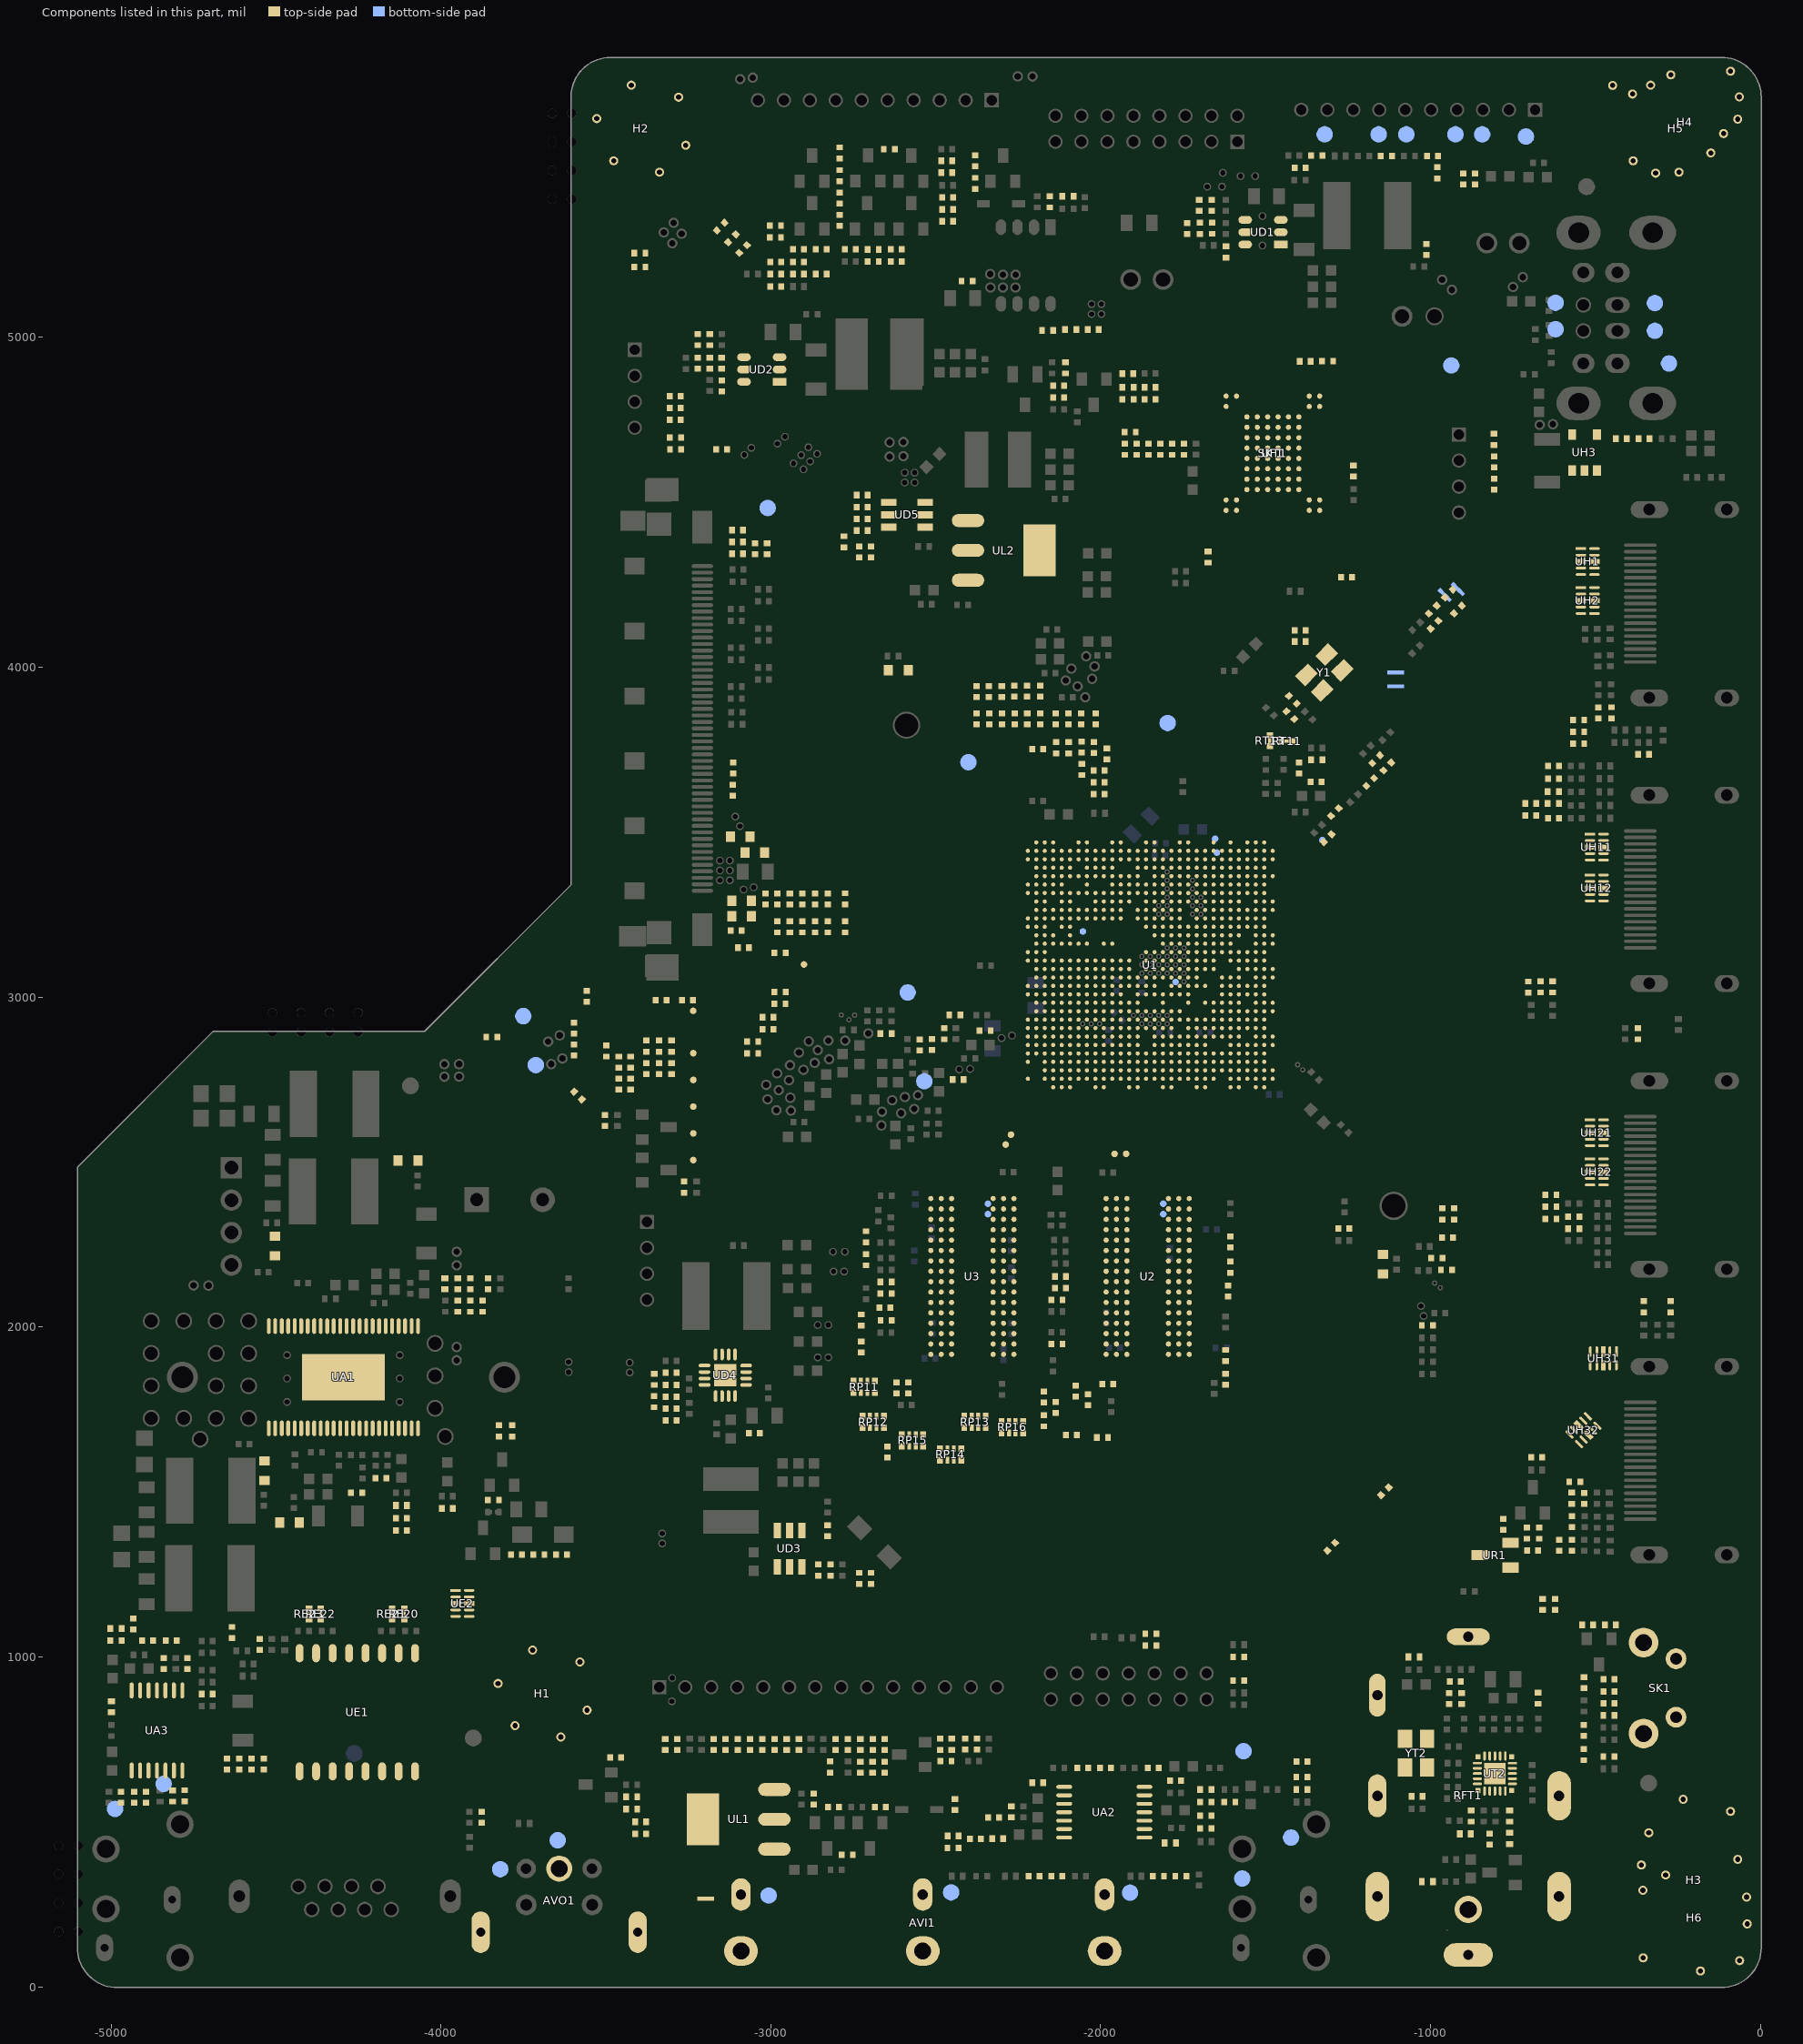
[diagram p0: the components of this part, seen from the top]
# Altium PCB MISC86290.PcbDoc (part 4 of 31)
Units mil, origin at the board's own origin, x right, y up, seen from the top; angles counter-clockwise.
Board outline 5104.71 x 5851.49 mil, 2 copper layers (TopLayer, BottomLayer), stack 61.855 mil thick; 1026 components, 667 nets, 4280 pads, 2294 vias.

## Components (designator, comment, footprint, x,y, rotation, side; value= is the part's Value field where it differs from the comment) (continued)
RE3 "75ohm-0402-±1%-1/16W" R0402 -4611.33,675.23 r270 top
RE4 "75ohm-0402-±1%-1/16W" R0402 -4648.5,675.23 r270 top
RE6 "0ohm-0402-±5%-1/16W" R0402 -4549.6,1037.94 r270 top
RE20 "NC/0ohm-0402-PCB" R0402SC -4111.5,1130.02 r270 top
RE21 "NC/0ohm-0402-PCB" R0402SC -4148.5,1130.02 r270 top
RE22 "NC/0ohm-0402-PCB" R0402SC -4364.5,1130.02 r270 top
RE23 "NC/0ohm-0402-PCB" R0402SC -4400,1130.02 r270 top
RF1 "Thick-film resistor,RES,1/16W,1Kohm,±5%,0402,SMD" R0402 -1910.52,4713.11 r180 top
RF2 "Thick-film resistor,RES,1/16W,3.9Kohm,±1%,0402,SMD" R0402 -1234,4594.77 r270 top
RF3 "0ohm-0402-±5%-1/16W" R0402 -1783.25,4660.84 r90 top
RF4 "0ohm-0402-±5%-1/16W" R0402 -1819.25,4660.84 r90 top
RF5 "0ohm-0402-±5%-1/16W" R0402 -1891.25,4660.84 r90 top
RF6 "0ohm-0402-±5%-1/16W" R0402 -1747.25,4660.84 r90 top
RF7 "0ohm-0402-±5%-1/16W" R0402 -1855.25,4660.84 r90 top
RF8 "0ohm-0402-±5%-1/16W" R0402 -1927.25,4660.84 r90 top
RF56 "Thick-film resistor,RES,1/16W,300Kohm,±1%,0402,SMD" R0402 -1917.25,4848.95 r180 top
RFT1 "RF shield can,RF SHLED,Single,H,F,T14.5,CH6.3,whole,25.0×14.5×10.0mm,DIP,T-14.5×25×10-F14.5-LHD (integrated),LHD" T-14.5×25×10-F14.5-2 -885.83,98.43 r0 top locked
RG1 "NC/1Kohm-0402-±5%-1/16W" R0402 -2464.25,5352 r0 top
RG2 "NC/4K7ohm-0402-±5%-1/16W" R0402 -2847,5267 r180 top
RG3 "NC/33ohm-0402-±5%-1/16W" R0402 -2464.25,5387.84 r180 top
RG4 "4K7ohm-0402-±5%-1/16W" R0402 -2464.25,5424.84 r0 top
RG5 "100ohm-0402-±5%-1/16W" R0402 -2847,5192 r180 top
RG6 "NC/10Kohm-0402-±5%-1/16W" R0402 -3149.23,4661 r0 top
RG7 "NC/1Kohm-0402-±5%-1/16W" R0402 -2791,5354.5 r270 top
RG8 "NC/10Kohm-0402-±5%-1/16W" R0402 -2689.5,5266.5 r180 top
RG11 "NC/10Kohm-0402-±5%-1/16W" R0402 -2986,5303.5 r180 top
RG12 "NC/1Kohm-0402-±5%-1/16W" R0402 -2620,5230.5 r0 top
RG13 "NC/33ohm-0402-±5%-1/16W" R0402 -2467,5499.5 r0 top
RG14 "4K7ohm-0402-±5%-1/16W" R0402 -2467,5535.5 r180 top
RG15 "100ohm-0402-±5%-1/16W" R0402 -2986,5339.5 r180 top
RG16 "NC/10Kohm-0402-±5%-1/16W" R0402 -3557.76,3002.2 r270 top
RG17 "NC/1Kohm-0402-±5%-1/16W" R0402 -2791,5559.5 r270 top
RG18 "NC/10Kohm-0402-±5%-1/16W" R0402 -2641,5571 r180 top
RG30 "NC/4K7ohm-0402-±5%-1/16W" R0402 -2985,5229 r180 top
RG31 "4K7ohm-0402-±5%-1/16W" R0402 -2916,5192 r180 top
RG32 "NC/100ohm-0402-±5%-1/16W" R0402 -2985,5154 r0 top
RG33 "100ohm-0402-±5%-1/16W" R0402 -2985,5192 r0 top
RG34 "NC/10Kohm-0402-±5%-1/16W" R0402 -2916,5229 r180 top
RG35 "0ohm-0402-±5%-1/16W" R0402 -2916,5267 r180 top
RG36 "NC/10Kohm-0402-±5%-1/16W" R0402 -2791,5422.5 r90 top
RG37 "NC/1Kohm-0402-±5%-1/16W" R0402 -2620,5267 r0 top
RG38 "NC/1Kohm-0402-±5%-1/16W" R0402 -2791,5490.5 r90 top
RG39 "NC/33ohm-0402-±5%-1/16W" R0402 -2689.5,5230 r180 top
RG40 "NC/2K2ohm-0402-±5%-1/16W" R0402 -2759,5267 r0 top
RG41 "100ohm-0402-±5%-1/16W" R0402 -3152,5336 r225 top
RG42 "100ohm-0402-±5%-1/16W" R0402 -3084,5268 r225 top
RG43 "100ohm-0402-±5%-1/16W" R0402 -2972,3134.5 r0 top
RG44 "100ohm-0402-±5%-1/16W" R0402 -3289.27,4696.5 r0 top
RH1 "Thick-film resistor,RES,1/16W,33ohm,±5%,0402,SMD" R0402 -354,3736 r180 top
RH2 "47Kohm-0402-±5%-1/16W" R0402 -451,3862 r270 top
RH3 "47Kohm-0402-±5%-1/16W" R0402 -491,3861.73 r270 top
RH4 "Thick-film resistor,RES,1/16W,33ohm,±5%,0402,SMD" R0402 -551,3768 r0 top
RH5 "100ohm-0402-±5%-1/16W" R0402 -551,3840 r180 top
RH6 "100ohm-0402-±5%-1/16W" R0402 -551,3804 r180 top
RH11 "Thick-film resistor,RES,1/16W,33ohm,±5%,0402,SMD" R0402 -627,3701 r0 top
RH12 "Thick-film resistor,RES,1/16W,33ohm,±5%,0402,SMD" R0402 -627,3662 r0 top
RH13 "47Kohm-0402-±5%-1/16W" R0402 -628,3623 r180 top
RH14 "47Kohm-0402-±5%-1/16W" R0402 -628,3587 r180 top
RH15 "100ohm-0402-±5%-1/16W" R0402 -696,3551 r180 top
RH16 "100ohm-0402-±5%-1/16W" R0402 -696,3587 r180 top
RH17 "Thick-film resistor,RES,1/16W,100ohm,±5%,0402,SMD" R0402 -627,3542 r180 top
RH21 "Thick-film resistor,RES,1/16W,33ohm,±5%,0402,SMD" R0402 -635,2328 r0 top
RH22 "Thick-film resistor,RES,1/16W,33ohm,±5%,0402,SMD" R0402 -372,2889 r270 top
RH23 "47Kohm-0402-±5%-1/16W" R0402 -566,2298 r0 top
RH24 "47Kohm-0402-±5%-1/16W" R0402 -566,2334 r0 top
RH25 "100ohm-0402-±5%-1/16W" R0402 -635,2401 r180 top
RH26 "100ohm-0402-±5%-1/16W" R0402 -635,2365 r180 top
RH31 "Thick-film resistor,RES,1/16W,33ohm,±5%,0402,SMD" R0402 -610,1338 r270 top
RH32 "Thick-film resistor,RES,1/16W,33ohm,±5%,0402,SMD" R0402 -571,1338 r90 top
RH33 "47Kohm-0402-±5%-1/16W" R0402 -572,1481 r90 top
RH34 "47Kohm-0402-±5%-1/16W" R0402 -534,1480 r270 top
RH35 "100ohm-0402-±5%-1/16W" R0402 -563,1531 r180 top
RH36 "100ohm-0402-±5%-1/16W" R0402 -571,1410 r270 top
RH37 "100ohm-0402-±5%-1/16W" R0402 -272,2061.5 r90 top
RH38 "100ohm-0402-±5%-1/16W" R0402 -353.77,2061.5 r90 top
RI1 "33ohm-0402-±5%-1/16W" R0402 -1183,3652 r225 top
RI2 "75ohm-0402-±5%-1/16W" R0402 -1131,3699 r225 top
RI3 "10Kohm-0402-±5%-1/16W" R0402 -2202,335 r0 top
RI4 "18Kohm-0402-±1%-1/16W" R0402 -2133.27,335 r180 top
RI5 "18Kohm-0402-±1%-1/16W" R0402 -1757,335 r180 top
RI6 "10Kohm-0402-±5%-1/16W" R0402 -1825,335 r0 top
RI115 "NC/0ohm-0402-±5%-1/16W" R0402 -1165,3721 r225 top
RI116 "NC/SHORT" GND -3197.65,267 r0 top
RK1 "4K7ohm-0402-±5%-1/16W" R0402 -2728.5,665.5 r270 top
RK2 "1Kohm-0402-±5%-1/16W" R0402 -2728.5,734 r270 top
RK10 "NC/1Kohm-0402-±5%-1/16W" R0402 -2655,665 r270 top
RK13 "NC/33Kohm-0402-±5%-1/16W" R0402 -2451.5,735 r270 top
RK14 "NC/510ohm-0402-±1%-1/16W" R0402 -2410.5,735.5 r90 top
RK15 "10Kohm-0402-±5%-1/16W" R0402 -2487,735 r90 top
RK23 "22ohm-0402-±5%-1/16W" R0402 -2469,684 r0 top
RK24 "1Kohm-0402-±1%-1/16W" R0402 -2820,666 r270 top
RK26 "1Kohm-0402-±5%-1/16W" R0402 -2803.64,734.27 r270 top
RK27 "NC/200ohm-0402-±1%-1/16W" R0402 -2951.94,734.27 r90 top
RK28 "NC/0ohm-0402-±5%-1/16W" R0402 -2989,734.27 r90 top
RK29 "NC/2K2ohm-0402-±1%-1/16W" R0402 -3026.07,734.27 r90 top
RK30 "NC/1Kohm-0402-±1%-1/16W" R0402 -3063.13,734.27 r270 top
RK31 "NC/470ohm-0402-±1%-1/16W" R0402 -3100.19,734.27 r90 top
RK32 "NC/0ohm-0402-±5%-1/16W" R0402 -3172.88,734.27 r90 top
RK33 "1Kohm-0402-±5%-1/16W" R0402 -3284.06,734.27 r270 top
RK34 "1Kohm-0402-±1%-1/16W" R0402 -3320.25,734.27 r270 top
RK35 "0ohm-0402-±5%-1/16W" R0402 -2914.88,734.27 r90 top
RK36 "0ohm-0402-±5%-1/16W" R0402 -3137.25,734.27 r90 top
RK37 "NC/0ohm-0402-±5%-1/16W" R0402 -2655,734 r270 top
RK38 "0ohm-0402-±5%-1/16W" R0402 -2375,735.5 r270 top
RK40 "NC/0ohm-0402-±5%-1/16W" R0402 -2691,734 r90 top
RK41 "NC/0ohm-0402-±5%-1/16W" R0402 -2766.5,734.5 r90 top
RK42 "510ohm-0402-±1%-1/16W" R0402 -2691.5,665.5 r270 top
RM1 "15Kohm-0402-±1%-1/16W" R0402 -1917.52,4890 r0 top
RM2 "4K7ohm-0402-±5%-1/16W" R0402 -2107,4907.54 r270 top
RM3 "47Kohm-0402-±5%-1/16W" R0402 -2127.5,4854 r180 top
RM4 "1Kohm-0402-±5%-1/16W" R0402 -2127.5,4817.5 r0 top
RM11 "4K7ohm-0402-±5%-1/16W" R0402 -2380.81,5467.12 r270 top
RM12 "10Kohm-0402-±5%-1/16W" R0402 -2381,5535.5 r270 top
RM13 "4K7ohm-0402-±5%-1/16W" R0402 -2099.25,5428 r180 top
RM14 "47Kohm-0402-±5%-1/16W" R0402 -2154.25,5411 r270 top
RM15 "NC/4K7ohm-0402-±5%-1/16W" R0402 -2405.25,5171 r180 top
RO1 "100ohm-0402-±5%-1/16W" R0402 -981,2208.5 r0 top
RO2 "NC/120ohm-0402-±5%-1/16W" R0402 -951.77,2173 r180 top
RO3 "0ohm-0402-±5%-1/16W" R0402 -3876.25,513.27 r270 top
RO11 "10Kohm-0402-±5%-1/16W" R0402 -1840.5,663.01 r180 top
RO12 "10Kohm-0402-±5%-1/16W" R0402 -1608.5,559.5 r180 top
RO13 "10Kohm-0402-±5%-1/16W" R0402 -1985.5,663.01 r180 top
RO14 "10Kohm-0402-±5%-1/16W" R0402 -1681.5,597.86 r180 top
RO15 "5R1ohm-0402-±5%-1/16W" R0402 -1390.4,635.36 r0 top
RO16 "5R1ohm-0402-±5%-1/16W" R0402 -1681.5,518 r0 top
RO17 "NC/SHORT" GND -1105.84,3942 r180 bottom
RO18 "NC/SHORT" GND -1105.84,3984 r180 bottom
RO19 "NC/?" R0402 -2447.73,457 r180 top
RO20 "1Kohm-0402-±5%-1/16W" R0402 -2379.73,448 r0 top
RO21 "30Kohm-0402-±1%-1/16W" R0402 -2312,449 r0 top
RO22 "1Kohm-0402-±5%-1/16W" R0402 -3470.27,695 r0 top
RO23 "10Kohm-0402-±5%-1/16W" R0402 -3394.73,500 r180 top
RO24 "1Kohm-0402-±5%-1/16W" R0402 -1390.4,597.86 r0 top
RO25 "1Kohm-0402-±5%-1/16W" R0402 -1681.5,480 r0 top
RO26 "10Kohm-0402-±5%-1/16W" R0402 -1390,682.5 r0 top
RO27 "4K7ohm-0402-±5%-1/16W" R0402 -3421.78,575.53 r0 top
RO28 "NC/?" R0402 -3421.78,538.53 r180 top
RO29 "0ohm-0402-±5%-1/16W" R0402 -2271,530 r90 top
RO30 "4K7ohm-0402-±5%-1/16W" R0402 -2325,513 r0 top
RO31 "47Kohm-0402-±1%-1/16W" R0402 -4768.34,980 r270 top
RO32 "47Kohm-0402-±1%-1/16W" R0402 -4708.52,887.15 r180 top
RO33 "100Kohm-0402-±1%-1/16W" R0402 -4840.84,980 r270 top
RO34 "100Kohm-0402-±1%-1/16W" R0402 -4894.5,574 r90 top
RO35 "NC/SHORT" GND -957,4219 r135 bottom
RO36 "NC/SHORT" GND -917,4237 r135 bottom
RO37 "5R1ohm-0402-±5%-1/16W" R0402 -4777,579 r270 top
RO38 "5R1ohm-0402-±5%-1/16W" R0402 -4930.5,574 r270 top
RO39 "NC/1Kohm-0402-±5%-1/16W" R0402 -4813.5,578 r270 top
RO40 "NC/1Kohm-0402-±5%-1/16W" R0402 -4969.75,573.94 r270 top
RO41 "NC/?" R0402 -4817.52,1049 r0 top
RO42 "30Kohm-0402-±1%-1/16W" R0402 -4985.16,1049 r180 top
RO43 "1Kohm-0402-±5%-1/16W" R0402 -4889.25,1049 r180 top
RO44 "0ohm-0402-±5%-1/16W" R0402 -4985.16,1086 r180 top
RO45 "4K7ohm-0402-±5%-1/16W" R0402 -4634,1074 r90 top
RO46 "1Kohm-0402-±5%-1/16W" R0402 -2448,421 r180 top
RO47 "1Kohm-0402-±5%-1/16W" R0402 -4933,1100 r90 top
RO51 "0ohm-0402-±5%-1/16W" R0402 -993.36,4174.81 r45 top
RO52 "0ohm-0402-±5%-1/16W" R0402 -988,4129 r45 top
RO53 "Thick-film resistor,RES,1/16W,200Kohm,±5%,0402,SMD" R0402 -944.57,4223.6 r225 top
RO54 "Thick-film resistor,RES,1/16W,200Kohm,±5%,0402,SMD" R0402 -917,4175 r225 top
RO55 "24Kohm-0402-±1%-1/16W" R0402 -2054.23,663 r180 top
RO56 "24Kohm-0402-±1%-1/16W" R0402 -1773,624.5 r180 top
RO57 "NC/47Kohm-0402-±5%-1/16W" R0402 -2191.23,618.5 r0 top
RO58 "NC/47Kohm-0402-±5%-1/16W" R0402 -1681.5,559.5 r180 top
RP1 "4K7ohm-0402-±5%-1/16W" R0402 -2022.5,5024 r0 top
RP5 "NC/4K7ohm-0402-±5%-1/16W" R0402 -2161,5021 r180 top
RP8 "100ohm-0402-±5%-1/16W" R0402 -2091,5024 r0 top
RP11 "Resistor array,RES ARRAY,1/16W,4×75ohm,±5%,0402,SMD" RA0402-MSD6886 -2717.11,1818.5 r270 top
RP12 "Resistor array,RES ARRAY,1/16W,4×75ohm,±5%,0402,SMD" RA0402-MSD6886 -2689.56,1712.2 r270 top
RP13 "Resistor array,RES ARRAY,1/16W,4×75ohm,±5%,0402,SMD" RA0402-MSD6886 -2381.22,1712.2 r270 top
RP14 "Resistor array,RES ARRAY,1/16W,4×75ohm,±5%,0402,SMD" RA0402-MSD6886 -2455.04,1613.78 r270 top
RP15 "Resistor array,RES ARRAY,1/16W,4×75ohm,±5%,0402,SMD" RA0402-MSD6886 -2570.46,1656.1 r270 top
RP16 "Resistor array,RES ARRAY,1/16W,4×75ohm,±5%,0402,SMD" RA0402-MSD6886 -2268.03,1696.46 r270 top
RR1 "1Kohm-0402-±5%-1/16W" R0402 -707.5,1375 r270 top
RR2 "10Kohm-0402-±5%-1/16W" R0402 -779.5,1401.27 r90 top
RR3 "4K7ohm-0402-±5%-1/16W" R0402 -535,922 r90 top
RR4 "2K2ohm-0402-±5%-1/16W" R0402 -455,1097 r0 top
RR5 "100ohm-0402-±5%-1/16W" R0402 -459,859.16 r180 top
RR6 "10Kohm-0402-±5%-1/16W" R0402 -2723.44,4485 r0 top
RR7 "10Kohm-0402-±5%-1/16W" R0402 -459,895.16 r180 top
RR8 "100ohm-0402-±5%-1/16W" R0402 -459.5,822.5 r180 top
RR9 "4K7ohm-0402-±5%-1/16W" R0402 -459,932 r180 top
RR10 "33ohm-0402-±5%-1/16W" R0402 -459.5,697.5 r0 top
RR11 "33ohm-0402-±5%-1/16W" R0402 -2442,552 r270 top
RR13 "4K7ohm-0402-±5%-1/16W" R0402 -2810.25,544.99 r180 top
RR14 "33ohm-0402-±5%-1/16W" R0402 -2870.25,569 r90 top
RR15 "4K7ohm-0402-±5%-1/16W" R0402 -2667.98,544.99 r180 top
RR16 "4K7ohm-0402-±5%-1/16W" R0402 -2768.25,400 r180 top
RR17 "10Kohm-0402-±5%-1/16W" R0402 -678.5,1605.5 r180 top
RR18 "NC/0ohm-0402-±5%-1/16W" R0402 -671,1375 r90 top
RR19 "NC/" R0402 -690.77,1322.5 r0 top
RT1 "0ohm-0402-±5%-1/16W" R0402 -1345,3719.5 r180 top
RT2 "100ohm-0402-±5%-1/16W" R0402 -535.5,776.73 r90 top
RT3 "0ohm-0402-±5%-1/16W" R0402 -820.89,447.37 r90 top
RT4 "Ferrite bead,BEAD,120ohm,0402,500mA,SMD,TP,GZ1005U121CTF,Sunlord" L0402 -1041,577 r0 top
RT5 "4K7ohm-0402-±5%-1/16W" R0402 -622.5,1158.78 r90 top
RT6 "4K7ohm-0402-±5%-1/16W" R0402 -660.5,1159.16 r90 top
RT7 "10Kohm-0402-±5%-1/16W" R0402 -1398.5,3695 r270 top
RT8 "100ohm-0402-±5%-1/16W" R0402 -535.5,703.5 r90 top
RT9 "100ohm-0402-±5%-1/16W" R0402 -674,874.5 r90 top
RT10 "100ohm-0402-±5%-1/16W" R0402 -943.82,873.61 r90 top
RT11 "NC/0ohm-0402-PCB" R0402SC -1435.5,3775.5 r180 top
RT12 "100ohm-0402-±5%-1/16W" R0402 -905.82,873.34 r90 top
RT13 "NC/0ohm-0402-PCB" R0402SC -1487.5,3777.23 r270 top
RT40 "NC/0ohm-0402-±5%-1/16W" R0402 -3394.52,463.15 r0 top
RU1 "0ohm-0402-±5%-1/16W" R0402 -964.6,2342.77 r270 top
RU2 "0ohm-0402-±5%-1/16W" R0402 -928.33,2342.75 r270 top
RU3 "4K7ohm-0402-±5%-1/16W" R0402 -353,4693 r0 top
RU5 "10Kohm-0402-±5%-1/16W" R0402 -2015,3844 r270 top
RU6 "4K7ohm-0402-±5%-1/16W" R0402 -422,4693 r180 top
RU7 "0ohm-0402-±5%-1/16W" R0402 -1395,4078 r0 top
RU8 "0ohm-0402-±5%-1/16W" R0402 -1395,4112 r0 top
RU9 "100ohm-0402-±5%-1/16W" R0402 -1981.5,3737.5 r90 top
RU10 "100ohm-0402-±5%-1/16W" R0402 -667,3031 r270 top
RU11 "NC/4K7ohm-0402-±5%-1/16W" R0402 -1345,5551 r0 top
RU12 "4K7ohm-0402-±5%-1/16W" R0402 -994.25,5550 r0 top
RU13 "0ohm-0402-±5%-1/16W" R0402 -865.15,5480.51 r270 top
RU14 "0ohm-0402-±5%-1/16W" R0402 -901.15,5480.51 r270 top
RU15 "100ohm-0402-±5%-1/16W" R0402 -980,5499 r270 top
RU16 "100ohm-0402-±5%-1/16W" R0402 -1134,5550 r0 top
RU17 "100ohm-0402-±5%-1/16W" R0402 -1395,5514 r0 top
RU18 "4K7ohm-0402-±5%-1/16W" R0402 -1254.77,4273 r180 top
RW1 "NC/NC/10Kohm-0402-±5%-1/16W" R0402 -3333,2991 r0 top
RW4 "NC/NC/4K7ohm-0402-±5%-1/16W" R0402 -3584.5,2701.5 r135 top
RW5 "NC/100ohm-0402-±5%-1/16W" R0402 -3101,4416 r180 top
RW8 "10Kohm-0402-±5%-1/16W" R0402 -3047.5,4359 r270 top
RW9 "10Kohm-0402-±5%-1/16W" R0402 -3011.5,4359 r270 top
RW10 "100ohm-0402-±5%-1/16W" R0402 -3100.78,4344 r0 top
RW11 "100ohm-0402-±5%-1/16W" R0402 -3100.98,4380 r0 top
RW26 "NC/0ohm-0402-±5%-1/16W" R0402 -3105.5,3202 r0 top
RW52 "NC/0ohm-0603-±5%-1/10W" R0603 -3088.5,3292.5 r0 top
RW53 "NC/0ohm-0603-±5%-1/10W" R0603 -3088.5,3245 r0 top
RW55 "0ohm-0603-±5%-1/10W" R0603 -3049,3438 r180 top
RW56 "0ohm-0603-±5%-1/10W" R0603 -3093,3486 r180 top
RW73 "NC/0ohm-0402-±5%-1/16W" R0402 -3083,3150 r0 top
RW251 "NC/4K7ohm-0402-±5%-1/16W" R0402 -2865.5,3213 r270 top
RW252 "NC/4K7ohm-0402-±5%-1/16W" R0402 -2865.5,3297.53 r90 top
RW389 "0ohm-0402-±5%-1/16W" R0402 -3016.5,3297.73 r90 top
RW393 "NC/33ohm-0402-±5%-1/16W" R0402 -3503,2626 r270 top
RW395 "NC/33ohm-0402-±5%-1/16W" R0402 -3263,2424 r90 top
RW405 "NC/4K7ohm-0402-±5%-1/16W" R0402 -2980.5,3213 r270 top
RW406 "NC/4K7ohm-0402-±5%-1/16W" R0402 -2942.5,3213 r270 top
RW407 "NC/4K7ohm-0402-±5%-1/16W" R0402 -2775,3213 r270 top
RW408 "NC/4K7ohm-0402-±5%-1/16W" R0402 -3115,3627 r270 top
RW409 "NC/4K7ohm-0402-±5%-1/16W" R0402 -2827.5,3213 r270 top
RW410 "NC/4K7ohm-0402-±5%-1/16W" R0402 -2904.34,3213 r270 top
RW412 "NC/4K7ohm-0402-±5%-1/16W" R0402 -2980.5,3297.53 r90 top
RW413 "NC/4K7ohm-0402-±5%-1/16W" R0402 -2942.5,3297.53 r90 top
RW414 "0ohm-0402-±5%-1/16W" R0402 -2775,3298 r90 top
RW415 "NC/4K7ohm-0402-±5%-1/16W" R0402 -3114,3695 r270 top
RW416 "NC/4K7ohm-0402-±5%-1/16W" R0402 -2827.5,3297.27 r90 top
RW417 "NC/4K7ohm-0402-±5%-1/16W" R0402 -2904.34,3297.27 r90 top
RW421 "NC/0ohm-0402-±5%-1/16W" R0402 -3252.5,2991 r180 top
S/N1 "Barcode" Barcode -3422,3927 r90 bottom
S/N2 "Barcode" Barcode -4264,1259 r0 bottom
SK1 "Tact switch,Tact Switch,160±50gf,7.0×10.3×7.0mm,DIP,106520070,VAST" KEY-HD-6 -157.48,905.51 r90 top locked
SKT1 "NC/SG-BGA-6367-TEST" TEST-SG-BGA-6367 -1477.51,4649.38 r180 top
SOC_RESETn "TEST" TP-20#1 -3235,2506 r90 top
U1 "TV main chip,IC Main Chip,MSDURN1801-R-00E3,64bit,Multi-Core,BGA758,SMD,Mstar" BGA758/0.65 -1849.72,3098.03 r180 top locked
U2 "DDR chip,IC DDR3,DDR3,2133M,16bit,256MB,2Gb,FBGA96,SMD,K4B2G1646F-BCNB,Samsung" BGA96/0.8-1 -1857.6,2153.15 r0 top locked
U3 "DDR chip,IC DDR3,DDR3,2133M,16bit,256MB,2Gb,FBGA96,SMD,K4B2G1646F-BCNB,Samsung" BGA96/0.8-1 -2389.09,2153.15 r0 top
UA1 "Audio amplifier,IC Audio AMP,Class D,2×20W@18V@8ohm,HTSSOP-48,SMD,TAS5751MDCAR,TI" SOP48/0.5-2 -4295.75,1847.75 r90 top
UA2 "Audio amplifier,IC Headphone AMP,Class AB,2×20mW@2.3V@32ohm,TSSOP-14,SMD,AD22653B-QH14NAR,ESMT" SSOP14/0.65-1 -1989,529 r270 top
UA3 "Audio amplifier,IC Headphone AMP,Class AB,2×20mW@2.3V@32ohm,TSSOP-14,SMD,AD22653B-QH14NAR,ESMT" SSOP14/0.65-1 -4860.92,776.77 r180 top
UD1 "DC-DC chip,IC DCDC,Syn,4A,17V,500KHz,SOT23-6,SMD,TPS564201,TI" SOP6/0.95 -1507.91,5318.92 r180 top locked
UD2 "DC-DC chip,IC DCDC,Syn,3A,17V,580KHz,TSOT23-6,SMD,TPS563201DDCR,TI" SOP6/0.95 -3027.41,4902.85 r180 top
UD3 "DC-DC chip,IC DCDC,Syn,2A,5.5V,1.5MHz,SOT23-6,SMD,TLV62569PDDCR,TI" SOT-23-6 -2943.25,1328 r180 top
UD4 "DC-DC chip,IC DC-DC,Syn,4A,5.5V,1.4MHz,VQFN-16,SMD,TLV62095RGTR,TI" QFN16/0.5-4 -3138.01,1853.69 r270 top
UD5 "DC-DC chip,IC DCDC,Syn,2A,5.5V,1.5MHz,SOT23-6,SMD,TLV62569PDDCR,TI" SOT-23-6 -2587,4462.5 r90 top
UE1 "Network transformer,Network Transformer,350uH,0.09×1P,H6.0MAX,H16101MC,SMD,MX" SOP16/1.27-2 -4253.5,832 r270 top locked
UE2 "NC/ULC0524P" RCL0524P -3935,1162 r270 top
UF1 "NAND FLASH chip,IC NAND FLASH,512MB,4Gb,SLC,P-TFBGA63,SMD,TC58NVG2S0HBAI4,Toshiba" BGA63/0.8-1 -1478,4648.89 r0 top
UH1 "NC/TVS diode,DIO ESD,0.4pF,19V,DFN2510-10L,SMD,ESD5304D-10/TR,Willsemi" RCL0524P -523.72,4320.31 r270 top
UH2 "NC/TVS diode,DIO ESD,0.4pF,19V,DFN2510-10L,SMD,ESD5304D-10/TR,Willsemi" RCL0524P -523.72,4202.37 r270 top
UH3 "Current-limit switch,IC OCP,2.1A,5.5V,H,SOT23-5,SMD,APL3551ABI-TRG,ANPEC" SOT-23-5 -533,4651 r0 top
UH11 "NC/TVS diode,DIO ESD,0.4pF,19V,DFN2510-10L,SMD,ESD5304D-10/TR,Willsemi" RCL0524P -496,3455 r270 top
UH12 "NC/TVS diode,DIO ESD,0.4pF,19V,DFN2510-10L,SMD,ESD5304D-10/TR,Willsemi" RCL0524P -496,3331 r270 top
UH21 "NC/TVS diode,DIO ESD,0.4pF,19V,DFN2510-10L,SMD,ESD5304D-10/TR,Willsemi" RCL0524P -496,2589 r270 top
UH22 "NC/TVS diode,DIO ESD,0.4pF,19V,DFN2510-10L,SMD,ESD5304D-10/TR,Willsemi" RCL0524P -496,2470 r270 top
UH31 "NC/TVS diode,DIO ESD,0.4pF,19V,DFN2510-10L,SMD,ESD5304D-10/TR,Willsemi" RCL0524P -476.26,1904.95 r180 top
UH32 "NC/TVS diode,DIO ESD,0.4pF,19V,DFN2510-10L,SMD,ESD5304D-10/TR,Willsemi" RCL0524P -536.56,1687.4 r225 top
UL1 "LC1117CLTR33" SOT-223 -3097.52,507.45 r90 top
UL2 "LDO chip,IC LDO,1A,1.2V,15V,SOT-223,SMD,LC1117CLTR12,Leadchip" SOT-223 -2294,4354.43 r270 top
UR1 "Reset IC,IC Reset,LOW,2.93V,SOT-23,SMD,SGM803-SXN3L/TR,SGMICRO" SOT-23-3-1 -804.5,1308.5 r90 top
UT2 "Silicon RF tuner,IC Si Tuner,QFN-24,SMD,SI2151-A10-GMR,Silicon Labs" QFN24/0.4-1 -804.89,646.37 r180 top locked
VCC_Panel "TEST" TP -3009.4,4483 r270 bottom
WAKE_ON_WIFIn "TEST" TP -1073.66,5615.53 r90 bottom locked
WIFI_DM "TEST" TP -843.66,5615.53 r90 bottom locked
WIFI_DP "TEST" TP -924.66,5615.53 r90 bottom locked
WIFI_REG_ON "TEST" TP -1157.37,5615.53 r90 bottom locked
XXXXXX "PCB_TIME" PCB_TIME -603,1751 r90 top
XXXXXXXXXXX "PCB_NAME" PCB_NAME -1198,1601 r90 top
Y1 "24MHz-±20ppm-16pF-3.2*2.5-SMD" XTAL-S-3 -1322.05,3984 r45 top
YT2 "24MHz-±20ppm-16pF-3.2*2.5-SMD" XTAL-S-3 -1044,708 r270 top

## Footprints (in the part's own frame and the unit in brackets; to place one, negate y for a bottom-side part, rotate by r counter-clockwise, add the part's x,y. Pads: shape width x height; smd on the part's side, far side on the other; paste and mask are expansions set on the pad)
AI_GRIPPER_V [mm] "3D shape for vertical type AI equipment"
  round 1.5 on Mech5: 0(0,-2.5) 1(0,0) 2(0,2.5)
  body extent -29.13,-4.7 2.5,4.7, height 54.74
ASSE3.5C-3#1 [mm] "定位孔(顶底层上锡)"
  round 3.5 on Keep-Out: 0(0,0)
  round 1.2 on Top Paste: 1(-2.443,-0.889) 1(-2.443,0.889) 1(-1.3,-2.252) 1(-1.3,2.252) 1(0.451,-2.56) 1(0.451,2.561) 1(1.992,-1.671) 1(1.992,1.671) 1(2.6,0)
  round 1.2 on Top Solder: 1(-2.443,-0.889) 1(-2.443,0.889) 1(-1.3,-2.252) 1(-1.3,2.252) 1(0.451,-2.56) 1(0.451,2.561) 1(1.992,-1.671) 1(1.992,1.671) 1(2.6,0)
  round 0.7 hole 0.4: 1(-2.3,-2.4) 2(-3.6,0.85) 3(-0.95,3.425) 4(2.7,2.5) 5(3.25,-1.2) 6(1.225,-3.275)
ASSE3.5C-3#2 [mm] "定位孔(顶底层上锡)"
  round 3.5 on Keep-Out: 0(0,0)
  round 1.2 on Top Paste: 1(-2.443,-0.889) 1(-2.443,0.889) 1(-1.3,-2.252) 1(0.451,-2.56) 1(1.992,-1.671) 1(2.6,0)
  round 1.2 on Top Solder: 1(-2.443,-0.889) 1(-2.443,0.889) 1(-1.3,-2.252) 1(0.451,-2.56) 1(1.992,-1.671) 1(2.6,0)
  round 0.7 hole 0.4: 1(-2.3,-2.4) 2(-3.6,0.85) 3(-0.95,3.425) 4(2.7,2.5) 5(3.25,-1.2) 6(1.225,-3.275)
ASSE3.5C-3#3 [mm] "定位孔(顶底层上锡)"
  round 3.5 on Keep-Out: 0(0,0)
  round 1.2 on Top Paste: 1(-2.443,-0.889) 1(-2.443,0.889) 1(-1.3,-2.252) 1(-1.3,2.252) 1(0.451,-2.56) 1(0.451,2.561) 1(1.992,-1.671) 1(1.992,1.671) 1(2.6,0)
  round 1.2 on Top Solder: 1(-2.443,-0.889) 1(-2.443,0.889) 1(-1.3,-2.252) 1(-1.3,2.252) 1(0.451,-2.56) 1(0.451,2.561) 1(1.992,-1.671) 1(1.992,1.671) 1(2.6,0)
  round 0.7 hole 0.4: 1(-2.3,-2.4) 2(-3.6,0.85) 3(-0.95,3.425) 4(2.7,2.5) 5(3.25,-1.2) 6(3.4,-8.993)
ASSE3.5C-3#4 [mm] "定位孔(顶底层上锡)"
  round 3.5 on Keep-Out: 0(0,0)
  round 0.7 hole 0.4: 1(-3.071,-5.351) 2(-4.849,0.745) 3(-1.903,2.218) 4(2.7,2.5) 5(3.25,-1.2) 6(2.161,-2.303)
  round 1.2 on Top Paste: 1(0.451,-2.56) 1(1.992,-1.671)
  round 1.2 on Top Solder: 1(0.451,-2.56) 1(1.992,-1.671)
ASSE3.5C-3#5 [mm] "定位孔(顶底层上锡)"
  round 3.5 on Keep-Out: 0(0,0)
  round 1.2 on Top Paste: 1(-2.443,-0.889) 1(-2.443,0.889) 1(-1.3,-2.252) 1(0.451,-2.56) 1(1.992,-1.671)
  round 1.2 on Top Solder: 1(-2.443,-0.889) 1(-2.443,0.889) 1(-1.3,-2.252) 1(0.451,-2.56) 1(1.992,-1.671)
  round 0.7 hole 0.4: 1(-2.3,-2.4) 2(-3.879,3.406) 3(-0.95,3.425) 4(5.881,2.517) 5(3.681,-1.793) 6(1.225,-3.275)
ASSE5.0C-3 [mm] "定位孔(顶底层上锡)"
  round 5 on Keep-Out mask+0: 0(0,0)
  round 0.7 hole 0.4: 1(-4.03,-2.778) 2(-4.054,2.425) 3(-4.169,4.373) 4(3.93,1.897) 5(3.983,-0.165) 6(0.382,-3.789)
  round 1.2 on Top Paste: 1(-2.585,2.169) 1(2.066,2.785) 1(3.17,1.154)
  round 1.2 on Top Solder: 1(-2.585,2.169) 1(2.066,2.785) 1(3.17,1.154)
AV1-H-4 [mm] "强生；AV38A-01S-5020;中心高度为5.5mm;14.08.09;170502更新信号脚孔径;170902更新接地脚宽度,17.12.29更新接地脚孔长度（18.05.07 更新地脚孔长度为2.5mm）"
  round 2 hole 1.3 mask+0.076: 1(0,8.05)
  round 2.2 on Top Overlay mask+0.076: 2(0,8.05)
  oval 1.4x3.2 hole 0.7 slot 2.5 at 90 deg mask+0.076: 2(6.05,3.15) 3(-6.05,3.15)
  oval 1.6x3.4 on Top Overlay mask+0.076: 3(-6.05,3.15) 3(6.05,3.15)
  silkscreen extent -6.4,0 6.4,8.7, body extent -7.25,-51.37 7.25,8.55, height 12.75
AV3-H14-15 [mm] "宇球；RC075-F03L3BY-A; 中心高度：5.5mm;15.11.24;170401兼容物料，更新高度;170802加大接地脚焊盘（18.03.09更新孔距）"
  oval 2.8x2.5 on Top Overlay: 0(-14,2.75) 0(0,2.75) 0(14,2.75)
  oval 1.7x2.7 on Top Overlay: 0(-14,7.1) 0(0,7.1) 0(14,7.1)
  oval 1.5x2.5 hole 0.8 slot 1.8 at 90 deg: 1(-14,7.1) 3(0,7.1) 5(14,7.1)
  oval 2.6x2.3 hole 1.3 slot 1.6 at 0 deg: 2(-14,2.75) 4(0,2.75) 6(14,2.75)
  silkscreen extent -20.3,0 20.3,7.8, body extent -20.1,-9 20.1,7.9, height 10.7
Barcode [mm]
  round 0.3 on Mech2: 0(0,0)
  silkscreen extent -14.62,-3.98 15.38,4.02
BGA63/0.8-1 [mm] "Spansion,S34ML01G200BHI000,17.02.06"
  round 0.4 smd: A1(-3.6,4.4) A2(-2.8,4.4) A9(2.8,4.4) A10(3.6,4.4) B1(-3.6,3.6) B9(2.8,3.6) B10(3.6,3.6) C3(-2,2.8) C4(-1.2,2.8) C5(-0.4,2.8) C6(0.4,2.8) C7(1.2,2.8) C8(2,2.8) D3(-2,2) D4(-1.2,2) D5(-0.4,2) D6(0.4,2) D7(1.2,2) D8(2,2) E3(-2,1.2) E4(-1.2,1.2) E5(-0.4,1.2) E6(0.4,1.2) E7(1.2,1.2) E8(2,1.2) F3(-2,0.4) F4(-1.2,0.4) F5(-0.4,0.4) F6(0.4,0.4) F7(1.2,0.4) F8(2,0.4) G3(-2,-0.4) G4(-1.2,-0.4) G5(-0.4,-0.4) G6(0.4,-0.4) G7(1.2,-0.4) G8(2,-0.4) H3(-2,-1.2) H4(-1.2,-1.2) H5(-0.4,-1.2) H6(0.4,-1.2) H7(1.2,-1.2) H8(2,-1.2) J3(-2,-2) J4(-1.2,-2) J5(-0.4,-2) J6(0.4,-2) J7(1.2,-2) J8(2,-2) K3(-2,-2.8) K4(-1.2,-2.8) K5(-0.4,-2.8) K6(0.4,-2.8) K7(1.2,-2.8) K8(2,-2.8) L1(-3.6,-3.6) L2(-2.8,-3.6) L9(2.8,-3.6) L10(3.6,-3.6) M1(-3.6,-4.4) M2(-2.8,-4.4) M9(2.8,-4.4) M10(3.6,-4.4)
  silkscreen extent -5.1,-5.5 4.5,6.12, body extent -4.5,-5.5 4.5,5.5, height 1